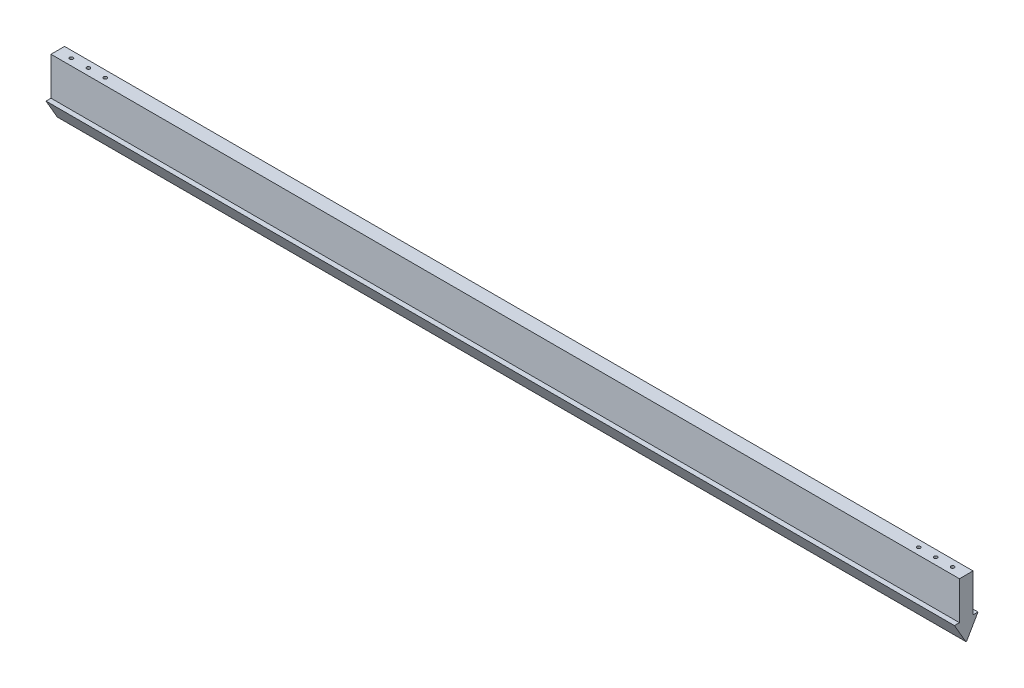
from build123d import *

# Parameters (mm, degrees)
EXTRUDE_1_DEPTH        = 1337
FILLET_1_R             = 1
HOLE_WIZARD_M6_1_D     = 5
HOLE_WIZARD_M6_1_DEPTH = 15
HOLE_WIZARD_M6_1_TIP   = 1.502151548


with BuildPart() as part:
    # 草图1 → 凸台-拉伸1 (new body)
    with BuildSketch(Plane(origin=(0, 0, 0), x_dir=(0, 0, -1), z_dir=(1, 0, 0))):
        Polygon((0, 0), (-17.320508076, 30), (-10, 30), (-10, 86), (10, 86), (10, 30), (17.320508076, 30), align=None)
    extrude(amount=EXTRUDE_1_DEPTH)

    # 圆角1
    fillet_1_edges = [part.edges().sort_by_distance(p)[0] for p in [
        (668.5, 0, 0),
    ]]
    fillet(fillet_1_edges, radius=FILLET_1_R)

    # M6 螺纹孔1
    with Locations(Plane(origin=(0, 86, 0), x_dir=(1, 0, 0), z_dir=(0, 1, 0))):
        with Locations((20, 0), (45, 0), (70, 0), (1317, 0), (1292, 0), (1267, 0)):
            Hole(HOLE_WIZARD_M6_1_D / 2, depth=HOLE_WIZARD_M6_1_DEPTH)
            with Locations((0, 0, -(HOLE_WIZARD_M6_1_DEPTH + HOLE_WIZARD_M6_1_TIP / 2))):  # 118° drill point
                Cone(0, HOLE_WIZARD_M6_1_D / 2, HOLE_WIZARD_M6_1_TIP, mode=Mode.SUBTRACT)


solid = part.part
